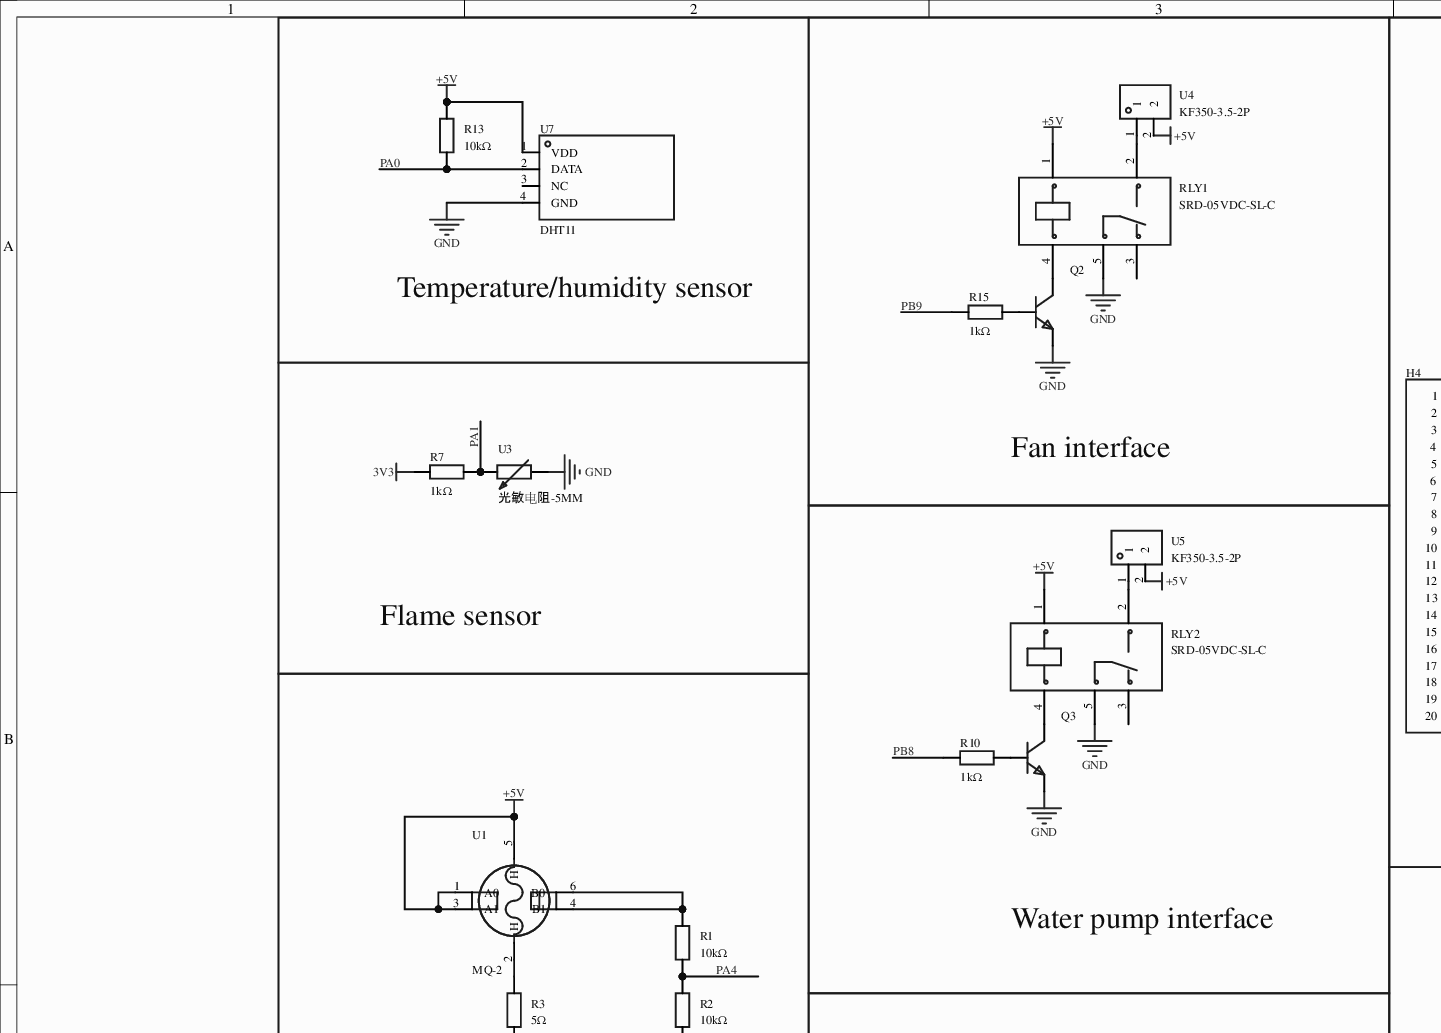
[diagram p0: MISC52121-3.schdoc, top left]
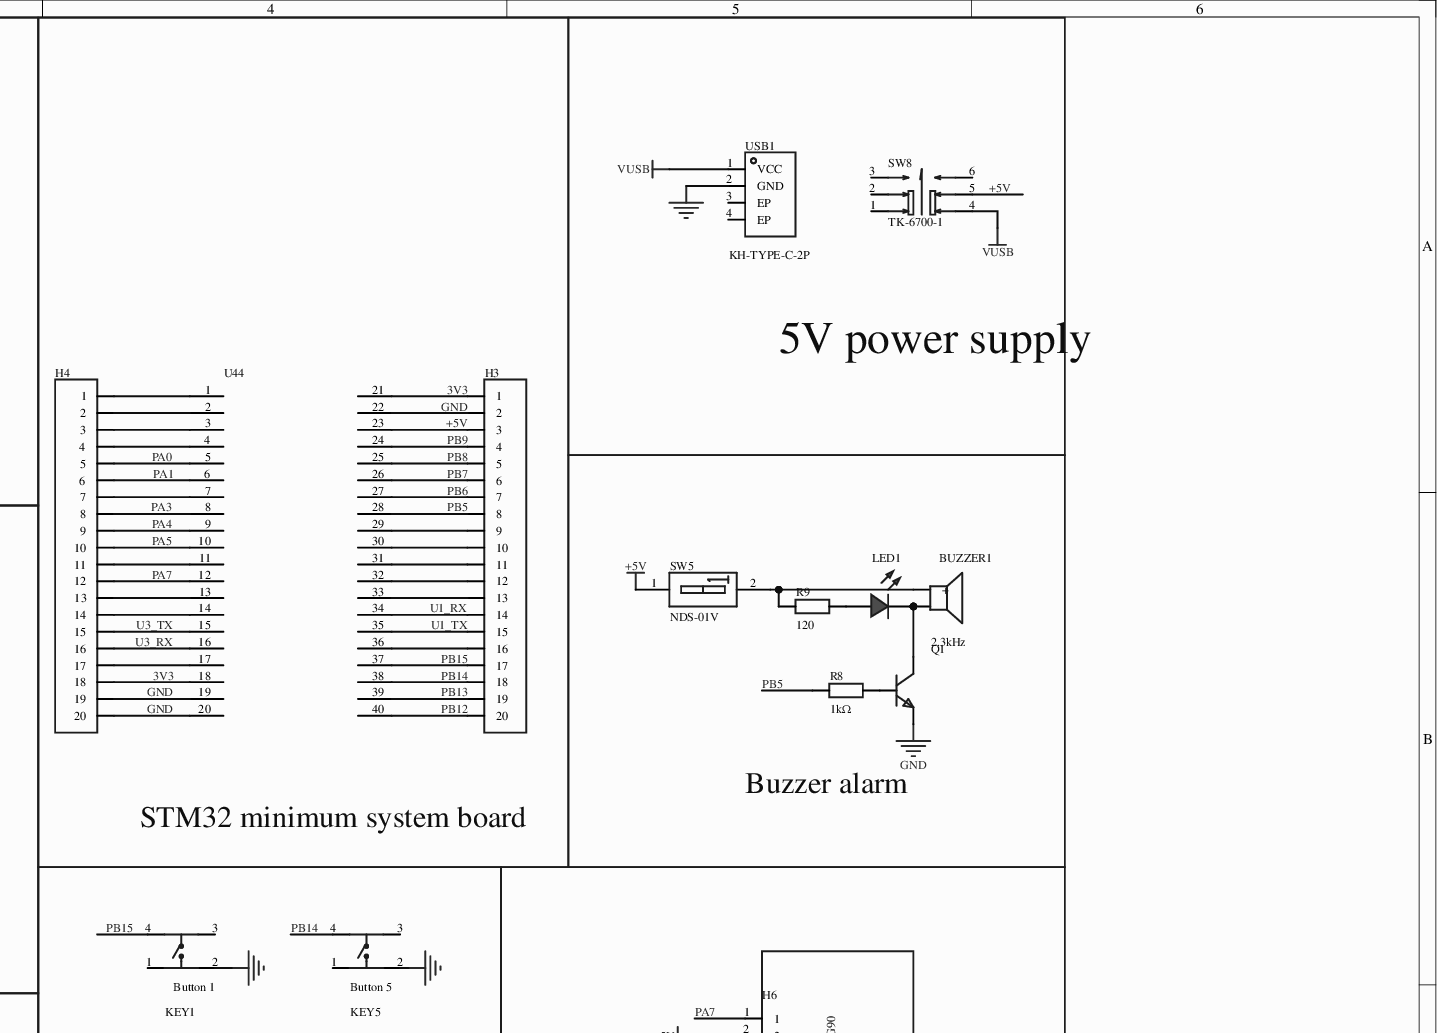
[diagram p1: MISC52121-3.schdoc, top right]
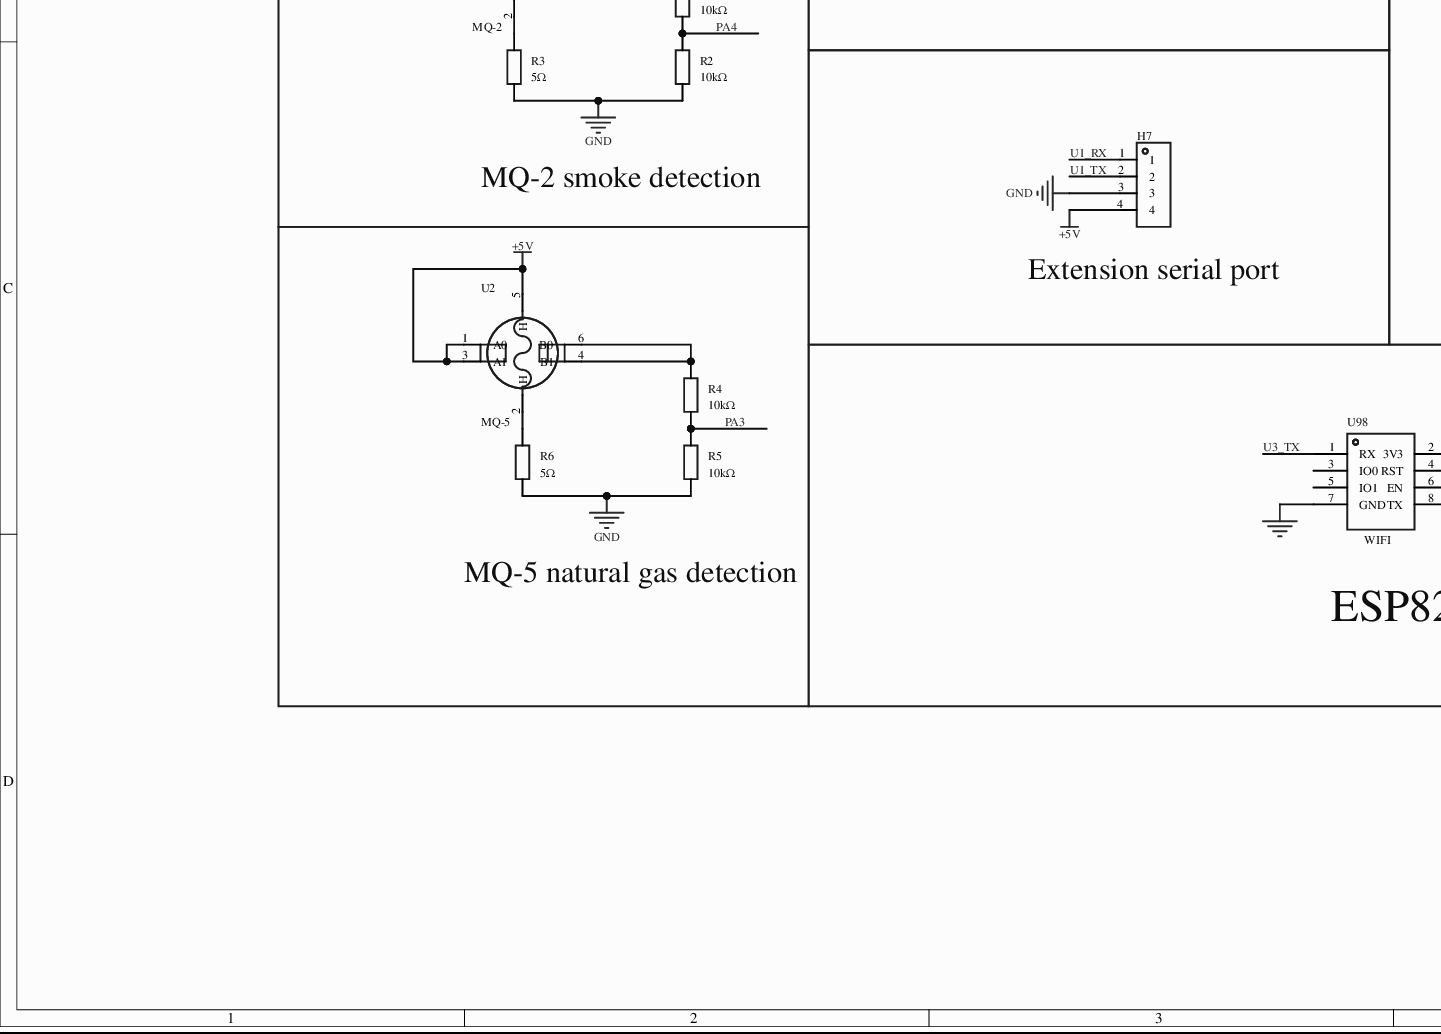
[diagram p2: MISC52121-3.schdoc, bottom left]
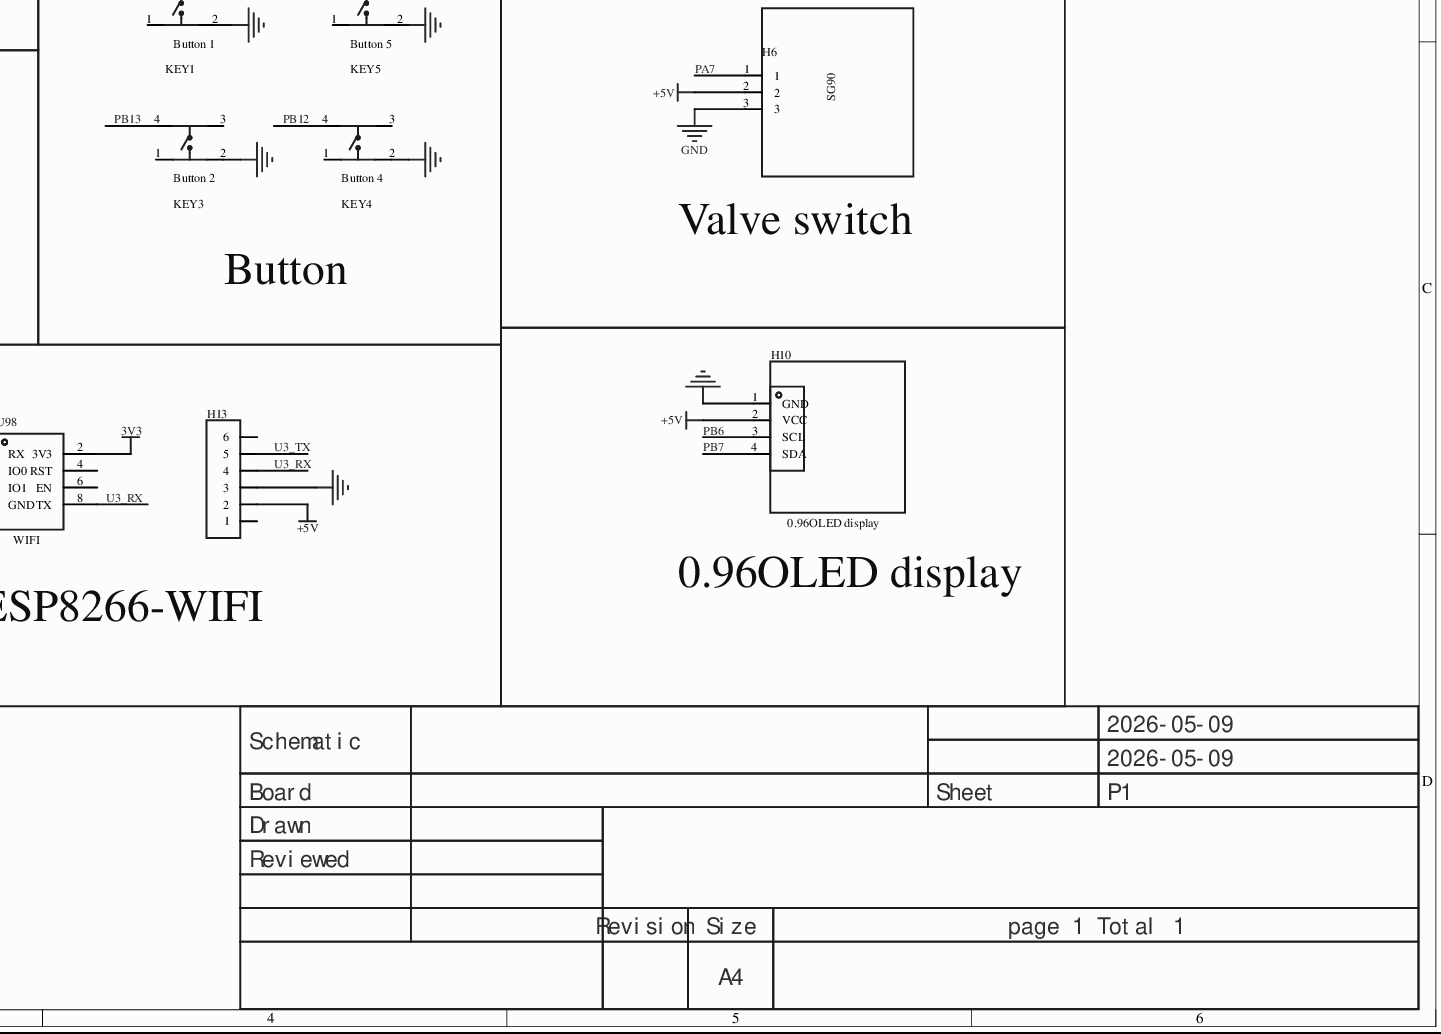
[diagram p3: MISC52121-3.schdoc, bottom right]
# Altium project MISC52121-2.PrjPcb
1 sheet, 40 parts. Net scope: global (net labels, ports and power ports of the same name join across sheets).
Board file: MISC52121.pcbdoc

## Sheet MISC52121-3.schdoc
size 420 x 297 mm; Version: V1.0; @Project Name: MISC52121; @Update Date: 2026-05-09; @Create Date: 2026-05-09; @Board Name: MISC52121; @Create Time: 16:45:37; @Page Count: 1; @Page No: 1; @Schematic Name: MISC52121; @Update Time: 16:45:37; Size: A4

### Parts
BUZZER1  2.3kHz  [BUZ-TH_BD12.0-P7.60-D0.6-FD]
H3  (no value)  [HDR-TH_20P-P2.54-V-F]
H4  (no value)  [HDR-TH_20P-P2.54-V-F]
H6  (no value)  [HDR-TH_3P-P2.54-V-F]
H7  (no value)  [HDR-TH_4P-P2.54-V-F]
H10  2.54-1*4P female  [HDR-TH_4P-P2.54-V-F]  (value not drawn)
H13  (no value)  [HDR-TH_6P-P2.54-V-M-1]
KEY1  Button 1  [KEY-TH_4P-L6.0-W6.0-P4.50-LS7.5]
KEY3  Button 2  [KEY-TH_4P-L6.0-W6.0-P4.50-LS7.5]
KEY4  Button 4  [KEY-TH_4P-L6.0-W6.0-P4.50-LS7.5]
KEY5  Button 5  [KEY-TH_4P-L6.0-W6.0-P4.50-LS7.5]
LED1  (no value)  [LED_TH-3mm]
Q1  (no value)  [S8050_TO_92]
Q2  (no value)  [S8050_TO_92]
Q3  (no value)  [S8050_TO_92]
R1  10kΩ  [Res_1/4W]
R2  10kΩ  [Res_1/4W]
R3  5Ω  [Res_1/4W]
R4  10kΩ  [Res_1/4W]
R5  10kΩ  [Res_1/4W]
R6  5Ω  [Res_1/4W]
R7  1kΩ  [Res_1/4W]
R8  1kΩ  [Res_1/4W]
R9  120  [Res_1/4W]
R10  1kΩ  [Res_1/4W]
R13  10kΩ  [Res_1/4W]
R15  1kΩ  [Res_1/4W]
RLY1  SRD-05VDC-SL-C  [RELAY-TH_SRD-XXVDC-XL-C]
RLY2  SRD-05VDC-SL-C  [RELAY-TH_SRD-XXVDC-XL-C]
SW5  NDS-01V  [SW-TH_2P-L3.9-W9.9-P2.54-LS7.6]
SW8  TK-6700-1  [SW-TH_TK-6700-1]
U1  MQ-2  [SENSOR-TH_MQ-2]
U2  MQ-5  [SENSOR-TH_MQ-2]
U3  光敏电阻-5MM  [RES-TH_L4.9-W4.3-P3.4]
U4  KF350-3.5-2P  [CONN-TH_P3.50_KF350-3.5-2P]
U5  KF350-3.5-2P  [CONN-TH_P3.50_KF350-3.5-2P]
U7  DHT11  [SENSOR-TH_DHT11]
U44  (no value)  [STM32最小系统板]
U98  (no value)  [WiFi封装]
USB1  KH-TYPE-C-2P  [USB-SMD_KH-TYPE-C-2P]

### Blocks framed on the sheet
Temperature/humidity sensor: R13 U7
Fan interface: Q2 R15 RLY1 U4
STM32 minimum system board: H3 H4 U44
5V power supply: SW8 USB1
Flame sensor: R7 U3
Buzzer alarm: BUZZER1 LED1 Q1 R8 R9 SW5
Water pump interface: Q3 R10 RLY2 U5
MQ-2 smoke detection: R1-R3 U1
Button: KEY1 KEY3-KEY5
Valve switch: H6
Extension serial port: H7
MQ-5 natural gas detection: R4-R6 U2
ESP8266-WIFI: H13 U98
0.96OLED display: H10

### Nets
3V3: H3.1 H4.18 R7.1 U44.18 U44.21 U98.2(3V3)
+5V: H3.3 H6.2 H7.4 H10.2(VCC) H13.2 R13.2 RLY1.1 RLY2.1 SW5.1(A1) SW8.5 U1.1(A0) U1.3(A1) U1.5(H) U2.1(A0) U2.3(A1) U2.5(H) U4.2 U5.2 U7.1(VDD) U44.23
GND: H3.2 H4.19 H4.20 H6.3 H7.3 H10.1(GND) H13.3 KEY1.2 KEY3.2 KEY4.2 KEY5.2 Q1.1(E) Q2.1(E) Q3.1(E) R2.1 R3.1 R5.1 R6.1 RLY1.5 RLY2.5 U3.1 U7.4(GND) U44.19 U44.20 U44.22 U98.7(GND) USB1.2(GND)
VUSB: SW8.4 USB1.1(VCC)
PA0: H4.5 R13.1 U7.2(DATA) U44.5
PA1: H4.6 R7.2 U3.2 U44.6
PA3: H4.8 R4.1 R5.2 U44.8
PA4: H4.9 R1.1 R2.2 U44.9
PA5: H4.10 U44.10
PA7: H4.12 H6.1 U44.12
PB5: H3.8 R8.1 U44.28
PB6: H3.7 H10.3(SCL) U44.27
PB7: H3.6 H10.4(SDA) U44.26
PB8: H3.5 R10.1 U44.25
PB9: H3.4 R15.1 U44.24
PB12: H3.20 KEY4.4 U44.40
PB13: H3.19 KEY3.4 U44.39
PB14: H3.18 KEY5.4 U44.38
PB15: H3.17 KEY1.4 U44.37
U1_RX: H3.14 H7.1 U44.34
U1_TX: H3.15 H7.2 U44.35
U3_RX: H4.16 H13.4 U44.16 U98.8(TX)
U3_TX: H4.15 H13.5 U44.15 U98.1(RX)
NetBUZZER1_1: BUZZER1.1(+) R9.1 SW5.2(A2)
NetBUZZER1_2: BUZZER1.2 LED1.2(A) Q1.3(C)
NetH3_9: H3.9 U44.29
NetH3_10: H3.10 U44.30
NetH3_11: H3.11 U44.31
NetH3_12: H3.12 U44.32
NetH3_13: H3.13 U44.33
NetH3_16: H3.16 U44.36
NetH4_1: H4.1 U44.1
NetH4_2: H4.2 U44.2
NetH4_3: H4.3 U44.3
NetH4_4: H4.4 U44.4
NetH4_7: H4.7 U44.7
NetH4_11: H4.11 U44.11
NetH4_13: H4.13 U44.13
NetH4_14: H4.14 U44.14
NetH4_17: H4.17 U44.17
NetLED1_1: LED1.1(C) R9.2
NetQ1_2: Q1.2(B) R8.2
NetQ2_2: Q2.2(B) R15.2
NetQ2_3: Q2.3(C) RLY1.4
NetQ3_2: Q3.2(B) R10.2
NetQ3_3: Q3.3(C) RLY2.4
NetR1_2: R1.2 U1.4(B1) U1.6(B0)
NetR3_2: R3.2 U1.2(H)
NetR4_2: R4.2 U2.4(B1) U2.6(B0)
NetR6_2: R6.2 U2.2(H)
NetRLY1_2: RLY1.2 U4.1
NetRLY2_2: RLY2.2 U5.1

Not connected (* = marked no-connect by the designer): H13 1 6; KEY1 1 3*; KEY3 1 3*; KEY4 1 3*; KEY5 1 3*; RLY1 3; RLY2 3; SW8 1* 2* 3* 6*; U7 3(NC); U98 3(IO0) 4(RST) 5(IO1) 6(EN); USB1 3(EP) 4(EP)

### Notes on the sheet
- 2026-05-09
- Schematic
- Board
- Sheet
- P1
- Drawn
- Reviewed
- Revision
- Size
- A4
- page 1 Total 1

### Library data of the parts
BUZZER1 = TMB12A05_C96093: Drive mode: active (built-in driver circuit); construction type: electromagnetic; rated voltage: 5V; frequency: 2.3kHz; sound pressure (SPL): 85dB@5V,10cm;; Manufacturer: 华能; 3D Model: 16ab50e14c5b4f2c986c135bdba60e37; 3D Model Transform: 472.44,472.176,0,90,0,0,-0.787,0,-177.165; Operating Voltage: 4V~8V; AddInBom: yes; ModelName: BUZ-TH_D12.0-H9.5-P7.60; Symbol: TMB12A05; Device: TMB12A05_C96093; LCSC Part Name: TMB12A05; Supplier Part: C96093; Manufacturer Part: TMB12A05; Supplier Footprint: 插件,D=12mm; JLCPCB Part Class: Extended Part; Datasheet: https://example.com/upload/public/pdf/source/20170522/1495448324811.pdf; Supplier: LCSC; Oscillator Circuit: Active (built-in driver circuit); Technology Type: Electromagnetic; Rated Voltage: 5V; Value: 2.3kHz; Sound Pressure Level (SPL): 85dB@5V,10cm; Diameter (φD): 12mm; Height: 9.8mm; ConvertToPcb: yes; FootprintName: BUZ-TH_BD12.0-P7.60-D0.6-FD
H3 H4 = HDR-F_2.54_1x20P: 3D Model: db7015f7ad9d48b8a3b1188db02e34290819f05c4eef4c71ace90d822a990e87; 3D Model Transform: 1999.996,100,0,0,0,0,0,0,-118.11; ConvertToPcb: yes; ModelName: HDR-F-2.54_1x20; Symbol: HDR-F_2.54_1x20P; Device: HDR-F_2.54_1x20P; Supplier Part: C50984; Supplier Footprint: 插件; AddInBom: yes; FootprintName: HDR-TH_20P-P2.54-V-F
H6 = HDR-F_2.54_1x3P: Symbol: PM254V-11-03-H85_1; 3D Model: f3b3cc5aae9641bf9e56fc160cef875b; 3D Model Transform: 299.9994,100,0,0,0,0,0,0,-118.11; ConvertToPcb: yes; ModelName: HDR2.54-F-LI-1X3P; Device: HDR-F_2.54_1x3P; Supplier Part: C541850; Supplier Footprint: 插件; AddInBom: yes; FootprintName: HDR-TH_3P-P2.54-V-F
H7 = HDR-F_2.54_1x4P: Symbol: 2.54-1*4P female; 3D Model: d187812051054f85879fcaa51a310d8e0819f05c4eef4c71ace90d822a990e87; 3D Model Transform: 419.6842,98.464,0,0,0,0,0,0,-118.11; ConvertToPcb: yes; Device: HDR-F_2.54_1x4P; Supplier Part: C2718488; Supplier Footprint: 插件; AddInBom: yes; FootprintName: HDR-TH_4P-P2.54-V-F; ModelName: HDR-TH_4P-P2.54-V-F
H10 = 0.96OLED屏幕: 插孔结构:1x4P;间距:2.54mm;行距:-;圆孔/方孔:方孔;安装类型:直插;排数:单排;总孔位数:4P;额定电流:3A;额定电压:-;插孔方向:顶部;塑高:-;触头材质:青铜;触头镀层:-;工作温度范围:-40℃~+105℃;焊接温度(最大值):-;; Manufacturer: BOOMELE(博穆精密); Manufacturer Part: 2.54-1*4P母; Symbol: 0.96OLED display; Holes Structure: 1x4P; Pitch: 2.54mm; Circular Hole / Square Hole: Square hole; Number of Holes: 4P; Current Rating (Max): 3A; Holes Direction: Top; 3D Model: 57daaad411c24bd7bd5d06edf5c4d16b; 3D Model Transform: 415.7472,98.425,0,0,0,0,0,0,-118.11; AddInBom: yes; ModelName: HDR-TH_4P-P2.54-F-LI-1X4P; Device: 0.96OLED display; Supplier: LCSC; Supplier Part: C2718488; JLCPCB Part Class: Extended library; LCSC Part Name: 间距:2.54mm 1x4P 直插; Supplier Footprint: 插件,P=2.54mm; Datasheet: https://example.com/upload/public/pdf/source/20210301/C2718488_F4427B881E42CAA8DDB0B1C12B3A522C.pdf; Row Spacing: -; Mounting Type: Through-hole; Number of Rows: Single row; Voltage Rating (Max): -; Insulation Height: -; Contact Material: Bronze; Contact Plating: -; Operating Temperature Range: -40℃~+105℃; Soldering Temperature(Max): -; ConvertToPcb: yes; FootprintName: HDR-TH_4P-P2.54-V-F
H13 = HDR-M_2.54_1x6P: Symbol: Header-Male-2.54_1x6; 3D Model: 60739dffc9b04830a286435b0fefbd4a; 3D Model Transform: 599.999,100,0,0,0,0,0,0,-118.11; ConvertToPcb: yes; ModelName: HDR2.54-M-LI-1X6P; Device: HDR-M_2.54_1x6P; Supplier Part: C37208; Supplier Footprint: 插件; AddInBom: yes; FootprintName: HDR-TH_6P-P2.54-V-M-1
KEY1 = 按键开关6*6*8: Circuit structure: SPST; contact rated current: -; button head type: Round Button; button actuation direction: Top Actuated;; Manufacturer Part: 按键1; Symbol: button6*6*8; Device: Tact switch 6*6*8; 3D Model: 84d39232fe0a426fa95ea2653754a6e5; 3D Model Transform: 306.868,236.22,0,0,0,0,0,0,-118.11; AddInBom: yes; ModelName: KEY-TH_4P-L6.0-W6.0-H4.5-LS6.5-P4.5; LCSC Part Name: 按键开关6*6*8   直插; Supplier Part: C59982; Supplier Footprint: Through Hole; JLCPCB Part Class: Extended library; Datasheet: https://example.com/upload/public/pdf/source/20151126/1457707591845.pdf; Supplier: LCSC; ConvertToPcb: yes; FootprintName: KEY-TH_4P-L6.0-W6.0-P4.50-LS7.5
KEY3 = 按键开关6*6*8: Circuit structure: SPST; contact rated current: -; button head type: Round Button; button actuation direction: Top Actuated;; Manufacturer Part: 按键2; Symbol: button6*6*8; Device: Tact switch 6*6*8; 3D Model: 84d39232fe0a426fa95ea2653754a6e5; 3D Model Transform: 306.868,236.22,0,0,0,0,0,0,-118.11; AddInBom: yes; ModelName: KEY-TH_4P-L6.0-W6.0-H4.5-LS6.5-P4.5; LCSC Part Name: 按键开关6*6*8   直插; Supplier Part: C59982; Supplier Footprint: Through Hole; JLCPCB Part Class: Extended library; Datasheet: https://example.com/upload/public/pdf/source/20151126/1457707591845.pdf; Supplier: LCSC; ConvertToPcb: yes; FootprintName: KEY-TH_4P-L6.0-W6.0-P4.50-LS7.5
KEY4 = 按键开关6*6*8: Circuit structure: SPST; contact rated current: -; button head type: Round Button; button actuation direction: Top Actuated;; Manufacturer Part: 按键4; Symbol: button6*6*8; Device: Tact switch 6*6*8; 3D Model: 84d39232fe0a426fa95ea2653754a6e5; 3D Model Transform: 306.868,236.22,0,0,0,0,0,0,-118.11; AddInBom: yes; ModelName: KEY-TH_4P-L6.0-W6.0-H4.5-LS6.5-P4.5; LCSC Part Name: 按键开关6*6*8   直插; Supplier Part: C59982; Supplier Footprint: Through Hole; JLCPCB Part Class: Extended library; Datasheet: https://example.com/upload/public/pdf/source/20151126/1457707591845.pdf; Supplier: LCSC; ConvertToPcb: yes; FootprintName: KEY-TH_4P-L6.0-W6.0-P4.50-LS7.5
KEY5 = 按键开关6*6*8: Circuit structure: SPST; contact rated current: -; button head type: Round Button; button actuation direction: Top Actuated;; Manufacturer Part: 按键5; Symbol: button6*6*8; Device: Tact switch 6*6*8; 3D Model: 84d39232fe0a426fa95ea2653754a6e5; 3D Model Transform: 306.868,236.22,0,0,0,0,0,0,-118.11; AddInBom: yes; ModelName: KEY-TH_4P-L6.0-W6.0-H4.5-LS6.5-P4.5; LCSC Part Name: 按键开关6*6*8   直插; Supplier Part: C59982; Supplier Footprint: Through Hole; JLCPCB Part Class: Extended library; Datasheet: https://example.com/upload/public/pdf/source/20151126/1457707591845.pdf; Supplier: LCSC; ConvertToPcb: yes; FootprintName: KEY-TH_4P-L6.0-W6.0-P4.50-LS7.5
LED1 = LED_TH-R_3mm: 3D Model: a497c992633541038a38947cdc58012f0819f05c4eef4c71ace90d822a990e87; 3D Model Transform: 141.274,153.327,0,0,0,0,-5.984,0,-137.795; ConvertToPcb: yes; ModelName: LED-TH-3mm_R; Symbol: LED_TH-R; Device: LED_TH-R_3mm; Supplier Footprint: 插件; AddInBom: yes; FootprintName: LED_TH-3mm
Q1-Q3 = S8050_TO_NPN: 3D Model: aafe8e06f2154e7c93506efd0d6632dd; 3D Model Transform: 180.78,141.44,417.3,0,0,0,0,0,-200; ConvertToPcb: yes; ModelName: TO-92-3_L4.9-W3.7-P1.27-L; Symbol: S8050_TO_NPN; Device: S8050_TO_NPN; Supplier Footprint: TO-92; AddInBom: yes; FootprintName: S8050_TO_92
R1-R6 R10 R13 R15 = Res_AXIAL-1/8W: Symbol: Resistor; 3D Model: b2b5ae7ae4c642178fe0039925c86a3f0819f05c4eef4c71ace90d822a990e87; 3D Model Transform: 282.86,66.88,253.09,0,0,0,0,0,-191; ConvertToPcb: yes; ModelName: RES-TH_BD1.8-L3.2-P7.20-D0.4; Device: Res_AXIAL-1/8W; Supplier Footprint: 轴向引线; AddInBom: yes; FootprintName: Res_1/4W
  R1 R2 R4 R5 R13: Value: 10kΩ
  R3 R6: Value: 5Ω
  R10 R15: Value: 1kΩ
R7 = Res_AXIAL-1/4W: Symbol: Resistor; 3D Model: 463263665006444ab7a47bd11b0cf9560819f05c4eef4c71ace90d822a990e87; 3D Model Transform: 427.165,94.32816,0,0,0,0,0,0,-196.85; AddInBom: yes; ModelName: RES-TH_BD2.4-L6.3-P10.30-D0.6; Device: Res_AXIAL-1/4W; Supplier Footprint: 轴向引线; Value: 1kΩ; ConvertToPcb: yes; FootprintName: Res_1/4W
R8 R9 = Res_AXIAL-1/4W: Symbol: Resistor; 3D Model: 463263665006444ab7a47bd11b0cf956; 3D Model Transform: 427.165,94.32816,0,0,0,0,0,0,-196.85; AddInBom: yes; ModelName: RES-TH_BD2.4-L6.3-P10.30-D0.6; Device: Res_AXIAL-1/4W; Supplier Footprint: 轴向引线; ConvertToPcb: yes; FootprintName: Res_1/4W
  R8: Value: 1kΩ
  R9: Value: 120
RLY1 RLY2 = SRD-05VDC-SL-C: Coil voltage: 5V; contact form: one changeover: 1C (SPDT); contact rating (resistive load): -; max switching voltage: 250V@AC; max switching current: 15A;; Manufacturer: 松乐; 3D Model: d0eda9b8bf8746d18ae810ab88dc78e70819f05c4eef4c71ace90d822a990e87; 3D Model Transform: 755.904,622.4397,0,0,0,0,34.882,0,-118.11; Coil Rated Power: 360mW; Coil Type: Non-polar, single coil; Coil Resistance: 70Ω; Contact Resistance: 100mΩ; Operate Time: 10ms; AddInBom: yes; ModelName: RELAY-TH_L19.2-W15.6-H15.8; Symbol: SRD-05VDC-SL-C; Device: SRD-05VDC-SL-C; LCSC Part Name: 蓝色 单组转换型继电器; Supplier Part: C35449; Manufacturer Part: SRD-05VDC-SL-C; Supplier Footprint: 插件,19.2x15.6mm; JLCPCB Part Class: Extended Part; Datasheet: https://example.com/datasheet/SRD-05VDC-SL-C/36422.html; Supplier: LCSC; Coil Voltage: 5V; Contact Form: One changeover: 1C (SPDT); Number of Pins: 5; Contact Rating: -; Switching Voltage(Max): 250V@AC; Switching Current(Max): 15A; Release Time: 10ms; ConvertToPcb: yes; FootprintName: RELAY-TH_SRD-XXVDC-XL-C
SW5 = NDS-01V_C501305: Forward-throw high lever; 3D Model: a6fe51954c31461ebc9e88beb6e51f3d0819f05c4eef4c71ace90d822a990e87; 3D Model Transform: 161.417,389.763,0,270,0,0,0,0,-125.984; AddInBom: yes; ModelName: SW-TH_L4.0-W9.9-H5.4-P2.54-B; Symbol: NDS-01V; Device: NDS-01V_C501305; LCSC Part Name: 拨码开关; Supplier Part: C501305; Manufacturer Part: NDS-01V; Supplier Footprint: DIP; JLCPCB Part Class: Extended Part; Supplier: LCSC; ConvertToPcb: yes; FootprintName: SW-TH_2P-L3.9-W9.9-P2.54-LS7.6
SW8 = TK-6700-1: Manufacturer: Yuandi(元迪); 3D Model: 1dccfbf2ceb24a728093c1f6ee61932a; 3D Model Transform: 275.59,275.59,0,90,0,0,0,0,-137.795; AddInBom: yes; Symbol: TK-6700-1; Device: TK-6700-1; LCSC Part Name: 自锁开关7*7*12.7有声有锁高导高柄插件双排6P按键开关带锁DIP六脚; Supplier Part: C528782; Manufacturer Part: TK-6700-1; Supplier Footprint: 插件; JLCPCB Part Class: Extended Part; Datasheet: https://example.com/upload/public/pdf/source/20200831/C528782_58F076EBF84BD8A9E2DE38DB1C0986D4.pdf; Supplier: LCSC; ConvertToPcb: yes; FootprintName: SW-TH_TK-6700-1; ModelName: SW-TH_TK-6700-1
U1 U2 = MQ-2: Manufacturer: Winsen(炜盛); 3D Model: a4c1c1cdd77042ea8ff9a8560a5de51a0819f05c4eef4c71ace90d822a990e87; 3D Model Transform: 747.59323,747.81158,0,0,0,0,0,0,-393.701; AddInBom: yes; Symbol: MQ-2; Device: MQ-2; LCSC Part Name: 可燃气体传感器; Supplier Part: C99296; Supplier Footprint: 插件; JLCPCB Part Class: Extended Part; Datasheet: https://example.com/upload/public/pdf/source/20180502/C99296_6F0BA5D7AA10C610B74ABFD8A5ECF346.pdf; Supplier: LCSC; ConvertToPcb: yes; FootprintName: SENSOR-TH_MQ-2; ModelName: SENSOR-TH_MQ-2
  U1: Manufacturer Part: MQ-2
  U2: Manufacturer Part: MQ-5
U3 = 光敏电阻-5MM: 3D Model: 8cda4899688949e78503a56fe341541c0819f05c4eef4c71ace90d822a990e87; 3D Model Transform: 169.291,200.6107,0,90,0,0,0,0,-196.85; AddInBom: yes; Symbol: 光敏电阻-5MM; Device: 光敏电阻-5MM; LCSC Part Name: 光敏电阻-5MM; Supplier Part: C9900003115; Manufacturer Part: 光敏电阻-5MM; Supplier Footprint: RES-TH_4.3X4.9X3.37P; JLCPCB Part Class: Extended Part; Supplier: LCSC; ConvertToPcb: yes; FootprintName: RES-TH_L4.9-W4.3-P3.4; ModelName: RES-TH_L4.9-W4.3-P3.4
U4 U5 = KF350-3.5-2P: 结构:1x2P;间距:3.5mm;颜色:绿色;安装方式:直插;额定电流:10A;额定电压:300V;排数:1;线规 - AWG:18~24;线规 - 平方毫米:0.75;每排PIN数:2;工作温度范围:-40℃~+105℃;; Manufacturer: KEFA(科发); 3D Model: b1d1e83e7d6a49aab33370f0163c64ca0819f05c4eef4c71ace90d822a990e87; 3D Model Transform: 314.96,271.653,0,0,0,0,0,1.968,-133.858; Structure: 1x2P; Pitch: 3.5mm; Current Rating (Max): 10A; Voltage Rating (Max): 300V; Wire Gauge - AWG: 18~24; Wire Gauge - mm2: 0.75; Number of PINs Per Row: 2; AddInBom: yes; Symbol: KF350-3.5-2P; Device: KF350-3.5-2P; LCSC Part Name: 3.5mm 1x2P 排数:1 每排P数:2 直插; Supplier Part: C474892; Manufacturer Part: KF350-3.5-2P; Supplier Footprint: 插件,P=3.5mm; JLCPCB Part Class: Extended Part; Datasheet: https://example.com/upload/public/pdf/source/20230317/986DB56DD49619EA586AA8816AA9D164.pdf; Supplier: LCSC; Color: Green; Mounting Style: Through-hole; Number of Pins: 2P; Number of Rows: 1; Operating Temperature Range: -40℃~+105℃; ConvertToPcb: yes; FootprintName: CONN-TH_P3.50_KF350-3.5-2P; ModelName: CONN-TH_P3.50_KF350-3.5-2P
U7 = DHT11: Temperature range: -20℃~+60℃; humidity range: 5%RH~95%RH; humidity accuracy: ±5%RH;; Manufacturer: 广州奥松; 3D Model: 6dde47d4d8bf4fa598dffcc067449c1d0819f05c4eef4c71ace90d822a990e87; 3D Model Transform: 236.25937,492.125,0,270,0,0,0,-11.811,-196.85; Voltage - Supply: 3.3V~5.5V; Current - Supply: 1mA; Temperature Tolerance: ±2℃; AddInBom: yes; Symbol: DHT11; Device: DHT11; LCSC Part Name: 新款电容式数字温湿度传感器,老款已停产16.1x12.6x5.8mm DHT11  电容式传感器; Supplier Part: C117051; Manufacturer Part: DHT11; Supplier Footprint: SIP-4; JLCPCB Part Class: Extended Part; Datasheet: https://example.com/datasheet/DHT11/118309.html; Supplier: LCSC; Temperature Range: -20℃~+60℃; Humidity: 5%RH~95%RH; Humidity Tolerance: ±5%RH; ConvertToPcb: yes; FootprintName: SENSOR-TH_DHT11; ModelName: SENSOR-TH_DHT11
U44 = STM32最小系统板: Symbol: STM32 minimum system board; AddInBom: yes; Device: STM32 minimum system board; ConvertToPcb: yes; FootprintName: STM32 minimum system board
U98 = WiFi模块: Symbol: WiFi module; AddInBom: yes; Device: WiFi module; ConvertToPcb: yes; FootprintName: WiFi footprint
USB1 = KH-TYPE-C-2P: Connector type: Type-C; standard: -; male/female: -; number of ports: -; number of contacts: 2P; mounting: -; rated current - power: -; contact material: -; contact plating: -; operating temperature range: -;; Manufacturer: kinghelm(金航标); 3D Model: 4464b34a7d0f48c2b8c2350e914c93f5; 3D Model Transform: 352.362,255.31449,0,0,0,0,0,-49.213,-98.425; Current Rating-Power: 3A; Voltage Rating: 20V; Connect-Disconnect Life: 5 thousand cycles; AddInBom: yes; Symbol: KH-TYPE-C-2P; Device: KH-TYPE-C-2P; LCSC Part Name: Type-C; Supplier Part: C2919656; Manufacturer Part: KH-TYPE-C-2P; Supplier Footprint: 插件; JLCPCB Part Class: Extended Part; Datasheet: https://example.com/upload/public/pdf/source/20220707/620587A9E0589B27D96D3CEE595CBC98.pdf; Supplier: LCSC; Connector Type: Type-C; Standard: -; Gender: -; Number of Ports: -; Number of Contacts: 2P; Mounting Style: -; Current Rating - Power (Max): -; Contact Material: -; Contact Plating: -; Operating Temperature Range: -; Protocol Standard: -; Mounting Type: Right-angle through-hole; Length: 6.43mm; Operating Temperature: -25℃~+85℃; ConvertToPcb: yes; FootprintName: USB-SMD_KH-TYPE-C-2P; ModelName: USB-SMD_KH-TYPE-C-2P